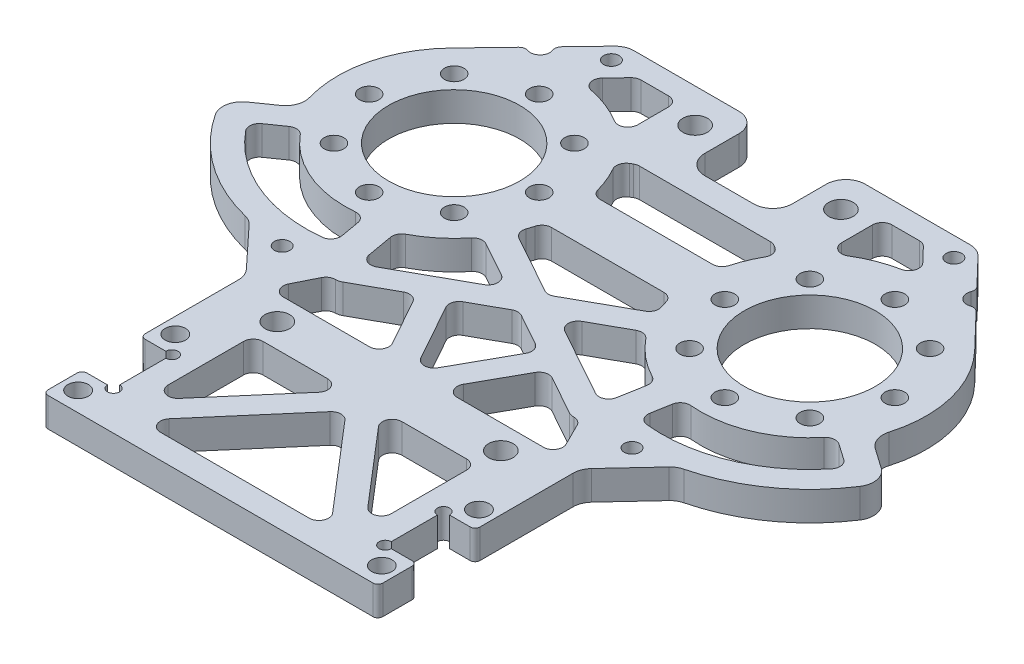
from build123d import *

# Parameters (mm, degrees)
SKETCH1_R              = 13.5
SKETCH1_R_2            = 2.525
SKETCH1_R_3            = 2.01
SKETCH1_R_4            = 2.1
SKETCH1_R_5            = 1.6
BOSS_EXTRUDE1_DEPTH    = 6
CUT_EXTRUDE1_DEPTH     = 111.547291087
R2_CUTOUT_FILLET_R     = 2
R1_PLUG_IN_FILLET_R    = 1
R4_OUTER_EDGE_FILLET_R = 4
F_73_20_MARKING_DEPTH  = 110.7530004


with BuildPart() as part:
    # Sketch1 → Boss-Extrude1 (new body)
    with BuildSketch(Plane(origin=(0, 0, 0), x_dir=(1, 0, 0), z_dir=(0, 1, 0))):
        with BuildLine():
            Line((-36.261062267, 35), (-9, 35))
            Line((-9, 35), (-9, 20))
            Line((-9, 20), (9, 20))
            Line((9, 20), (9, 35))
            Line((9, 35), (36.261062267, 35))
            Line((36.261062267, 35), (53.909452324, 16.624766472))
            ThreePointArc((53.909452324, 16.624766472), (60.203109588, 4.346632924), (58.696156922, -9.368022698))
            Line((58.696156922, -9.368022698), (68.25790113, -16.063228071))
            ThreePointArc((68.25790113, -16.063228071), (58.255238391, -28.130066659), (44.031297301, -34.713481825))
            Line((44.031297301, -34.713481825), (34.45, -45))
            Line((34.45, -45), (34.45, -66.75))
            Line((34.45, -66.75), (29.2, -66.75))
            ThreePointArc((29.2, -66.75), (27.066116524, -65.866116524), (27.95, -68))
            Line((27.95, -68), (27.95, -77.5))
            ThreePointArc((27.95, -77.5), (27.066116524, -79.633883476), (29.2, -78.75))
            Line((29.2, -78.75), (34.45, -78.75))
            Line((34.45, -78.75), (34.45, -86.75))
            Line((34.45, -86.75), (-34.45, -86.75))
            Line((-34.45, -86.75), (-34.45, -78.75))
            Line((-34.45, -78.75), (-29.2, -78.75))
            ThreePointArc((-29.2, -78.75), (-27.066116524, -79.633883476), (-27.95, -77.5))
            Line((-27.95, -77.5), (-27.95, -68))
            ThreePointArc((-27.95, -68), (-27.066116524, -65.866116524), (-29.2, -66.75))
            Line((-29.2, -66.75), (-34.45, -66.75))
            Line((-34.45, -66.75), (-34.45, -45))
            Line((-34.45, -45), (-44.031297301, -34.713481825))
            ThreePointArc((-44.031297301, -34.713481825), (-58.255238391, -28.130066659), (-68.25790113, -16.063228071))
            Line((-68.25790113, -16.063228071), (-58.696156922, -9.368022698))
            ThreePointArc((-58.696156922, -9.368022698), (-60.203109588, 4.346632924), (-53.909452324, 16.624766472))
            Line((-53.909452324, 16.624766472), (-36.261062267, 35))
        make_face()
        with Locations(Location((-36.6, 0, 0), (0, 0, 270))):
            Circle(SKETCH1_R, mode=Mode.SUBTRACT)
        with Locations(Location((-15, 28, 0), (0, 0, 270))):
            Circle(SKETCH1_R_2, mode=Mode.SUBTRACT)
        with Locations(Location((15, 28, 0), (0, 0, 270))):
            Circle(SKETCH1_R_2, mode=Mode.SUBTRACT)
        with Locations(Location((-23, -50, 0), (0, 0, 270))):
            Circle(SKETCH1_R_2, mode=Mode.SUBTRACT)
        with Locations(Location((23, -50, 0), (0, 0, 270))):
            Circle(SKETCH1_R_2, mode=Mode.SUBTRACT)
        with Locations(Location((36.6, 0, 0), (0, 0, 90))):
            Circle(SKETCH1_R, mode=Mode.SUBTRACT)
        with Locations(Location((-36.6, 17.5, 0), (0, 0, 270))):
            Circle(SKETCH1_R_3, mode=Mode.SUBTRACT)
        with Locations(Location((-24.225631329, 12.374368671, 0), (0, 0, 270))):
            Circle(SKETCH1_R_3, mode=Mode.SUBTRACT)
        with Locations(Location((-19.1, 0, 0), (0, 0, 270))):
            Circle(SKETCH1_R_3, mode=Mode.SUBTRACT)
        with Locations(Location((-24.225631329, -12.374368671, 0), (0, 0, 270))):
            Circle(SKETCH1_R_3, mode=Mode.SUBTRACT)
        with Locations(Location((-36.6, -17.5, 0), (0, 0, 270))):
            Circle(SKETCH1_R_3, mode=Mode.SUBTRACT)
        with Locations(Location((-48.974368671, -12.374368671, 0), (0, 0, 270))):
            Circle(SKETCH1_R_3, mode=Mode.SUBTRACT)
        with Locations(Location((-54.1, 0, 0), (0, 0, 270))):
            Circle(SKETCH1_R_3, mode=Mode.SUBTRACT)
        with Locations(Location((-48.974368671, 12.374368671, 0), (0, 0, 270))):
            Circle(SKETCH1_R_3, mode=Mode.SUBTRACT)
        with Locations(Location((48.974368671, 12.374368671, 0), (0, 0, 90))):
            Circle(SKETCH1_R_3, mode=Mode.SUBTRACT)
        with Locations(Location((54.1, 0, 0), (0, 0, 90))):
            Circle(SKETCH1_R_3, mode=Mode.SUBTRACT)
        with Locations(Location((48.974368671, -12.374368671, 0), (0, 0, 90))):
            Circle(SKETCH1_R_3, mode=Mode.SUBTRACT)
        with Locations(Location((36.6, -17.5, 0), (0, 0, 90))):
            Circle(SKETCH1_R_3, mode=Mode.SUBTRACT)
        with Locations(Location((24.225631329, -12.374368671, 0), (0, 0, 90))):
            Circle(SKETCH1_R_3, mode=Mode.SUBTRACT)
        with Locations(Location((19.1, 0, 0), (0, 0, 90))):
            Circle(SKETCH1_R_3, mode=Mode.SUBTRACT)
        with Locations(Location((24.225631329, 12.374368671, 0), (0, 0, 90))):
            Circle(SKETCH1_R_3, mode=Mode.SUBTRACT)
        with Locations(Location((36.6, 17.5, 0), (0, 0, 90))):
            Circle(SKETCH1_R_3, mode=Mode.SUBTRACT)
        with Locations(Location((-31.25, -82.75, 0), (0, 0, 270))):
            Circle(SKETCH1_R_4, mode=Mode.SUBTRACT)
        with Locations(Location((-31.25, -62.75, 0), (0, 0, 270))):
            Circle(SKETCH1_R_4, mode=Mode.SUBTRACT)
        with Locations(Location((31.25, -82.75, 0), (0, 0, 90))):
            Circle(SKETCH1_R_4, mode=Mode.SUBTRACT)
        with Locations(Location((31.25, -62.75, 0), (0, 0, 90))):
            Circle(SKETCH1_R_4, mode=Mode.SUBTRACT)
        with Locations(Location((-35.25, 31, 0), (0, 0, 270))):
            Circle(SKETCH1_R_5, mode=Mode.SUBTRACT)
        with Locations(Location((35.25, 31, 0), (0, 0, 90))):
            Circle(SKETCH1_R_5, mode=Mode.SUBTRACT)
        with Locations(Location((-36, -36, 0), (0, 0, 270))):
            Circle(SKETCH1_R_5, mode=Mode.SUBTRACT)
        with Locations(Location((36, -36, 0), (0, 0, 90))):
            Circle(SKETCH1_R_5, mode=Mode.SUBTRACT)
        with BuildLine():
            Line((-55.030920997, -12.905469818), (-61.584137351, -17.494081309))
            ThreePointArc((-61.584137351, -17.494081309), (-48.271844687, -28.178325742), (-31.303730581, -30.036636467))
            Line((-31.303730581, -30.036636467), (-32.692916002, -22.158174443))
            ThreePointArc((-32.692916002, -22.158174443), (-45.210377228, -20.787289482), (-55.030920997, -12.905469818))
        make_face(mode=Mode.SUBTRACT)
        with BuildLine():
            Line((55.030920997, -12.905469818), (61.584137351, -17.494081309))
            ThreePointArc((61.584137351, -17.494081309), (48.271844687, -28.178325742), (31.303730581, -30.036636467))
            Line((31.303730581, -30.036636467), (32.692916002, -22.158174443))
            ThreePointArc((32.692916002, -22.158174443), (45.210377228, -20.787289482), (55.030920997, -12.905469818))
        make_face(mode=Mode.SUBTRACT)
    extrude(amount=BOSS_EXTRUDE1_DEPTH)

    # Sketch3 → Cut-Extrude1 (cut, through all)
    with BuildSketch(Plane(origin=(0, 6, 0), x_dir=(1, 0, 0), z_dir=(0, 1, 0))):
        with BuildLine():
            Line((-35.748265569, 23.984881664), (-29.490856678, 30.5))
            Line((-29.490856678, 30.5), (-21, 30.5))
            Line((-21, 30.5), (-21, 18.238420984))
            ThreePointArc((-21, 18.238420984), (-27.886771893, 22.362460866), (-35.748265569, 23.984881664))
        make_face()
        with BuildLine():
            ThreePointArc((35.748265569, 23.984881664), (27.886771893, 22.362460866), (21, 18.238420984))
            Line((21, 18.238420984), (21, 30.5))
            Line((21, 30.5), (29.490856678, 30.5))
            Line((29.490856678, 30.5), (35.748265569, 23.984881664))
        make_face()
        with BuildLine():
            Line((-13.126610811, 5), (13.126610811, 5))
            ThreePointArc((13.126610811, 5), (14.513085915, 9.389793725), (16.712198489, 13.434111472))
            Line((16.712198489, 13.434111472), (14, 15))
            Line((14, 15), (-14, 15))
            Line((-14, 15), (-16.712198489, 13.434111472))
            ThreePointArc((-16.712198489, 13.434111472), (-14.513085915, 9.389793725), (-13.126610811, 5))
        make_face()
        with BuildLine():
            Line((13.126610811, -5), (-13.126610811, -5))
            ThreePointArc((-13.126610811, -5), (-13.719828244, -7.245532444), (-14.527321777, -9.423209435))
            ThreePointArc((-14.527321777, -9.423209435), (-14.469211894, -9.452626985), (-14.411888075, -9.483548344))
            Line((-14.411888075, -9.483548344), (0, -17.501639796))
            Line((0, -17.501639796), (14.411888075, -9.483548344))
            ThreePointArc((14.411888075, -9.483548344), (14.469211894, -9.452626985), (14.527321777, -9.423209435))
            ThreePointArc((14.527321777, -9.423209435), (13.719828244, -7.245532444), (13.126610811, -5))
        make_face()
        with BuildLine():
            ThreePointArc((-16.842763472, -13.852855474), (-16.899262321, -13.820451295), (-16.95489785, -13.786586289))
            ThreePointArc((-16.95489785, -13.786586289), (-21.266831345, -18.463313327), (-26.655934481, -21.842975094))
            Line((-26.655934481, -21.842975094), (-24.97170536, -31.394713087))
            Line((-24.97170536, -31.394713087), (-13.806916689, -25.183153842))
            Line((-13.806916689, -25.183153842), (-5.142180472, -20.362505289))
            Line((-5.142180472, -20.362505289), (-16.842763472, -13.852855474))
        make_face()
        with BuildLine():
            ThreePointArc((-23.296885286, -36.184653565), (-24.456132251, -36.499368441), (-25.628351624, -36.237069529))
            Line((-25.628351624, -36.237069529), (-30, -45))
            Line((-30, -45), (-5.642628511, -45))
            Line((-5.642628511, -45), (-13.560695072, -30.767898791))
            Line((-13.560695072, -30.767898791), (-23.296885286, -36.184653565))
        make_face()
        Polygon((9.191387942, -28.337023394), (0, -23.223370782), (-9.191387942, -28.337023394), (0, -44.857819528), align=None)
        with BuildLine():
            ThreePointArc((26.655934481, -21.842975094), (21.266831345, -18.463313327), (16.95489785, -13.786586289))
            ThreePointArc((16.95489785, -13.786586289), (16.899262321, -13.820451295), (16.842763472, -13.852855474))
            Line((16.842763472, -13.852855474), (5.142180472, -20.362505289))
            Line((5.142180472, -20.362505289), (13.806916944, -25.183153984))
            Line((13.806916944, -25.183153984), (24.97170536, -31.394713087))
            Line((24.97170536, -31.394713087), (26.655934481, -21.842975094))
        make_face()
        with BuildLine():
            Line((30, -45), (25.628351624, -36.237069529))
            ThreePointArc((25.628351624, -36.237069529), (24.456132251, -36.499368441), (23.296885286, -36.184653565))
            Line((23.296885286, -36.184653565), (13.560695072, -30.767898791))
            Line((13.560695072, -30.767898791), (5.642628511, -45))
            Line((5.642628511, -45), (30, -45))
        make_face()
        Polygon((-3.29399812, -55), (-22.95, -77.910590426), (-22.95, -55), align=None)
        Polygon((0, -58.839409574), (19.65600188, -81.75), (-19.65600188, -81.75), align=None)
        Polygon((22.95, -55), (3.29399812, -55), (22.95, -77.910590426), align=None)
    extrude(amount=-CUT_EXTRUDE1_DEPTH, mode=Mode.SUBTRACT)

    # R2 cutout fillet
    r2_cutout_fillet_edges = [part.edges().sort_by_distance(p)[0] for p in [
        (-13.126610811, 3, 5),
        (13.126610811, 3, 5),
        (26.655934481, 3, 21.842975094),
        (-26.655934481, 3, 21.842975094),
        (22.95, 3, 55),
        (22.95, 3, 77.910590426),
        (3.29399812, 3, 55),
        (19.65600188, 3, 81.75),
        (-19.65600188, 3, 81.75),
        (0, 3, 58.839409574),
        (-3.29399812, 3, 55),
        (-22.95, 3, 77.910590426),
        (-22.95, 3, 55),
        (-16.712198489, 3, -13.434111472),
        (14, 3, -15),
        (16.712198489, 3, -13.434111472),
        (13.126610811, 3, -5),
        (-13.126610811, 3, -5),
        (-14, 3, -15),
        (21, 3, -30.5),
        (29.490856678, 3, -30.5),
        (35.748265569, 3, -23.984881664),
        (21, 3, -18.238420984),
        (-5.142180472, 3, 20.362505289),
        (-24.97170536, 3, 31.394713087),
        (-16.95489785, 3, 13.786586289),
        (-14.527321777, 3, 9.423209435),
        (14.527321777, 3, 9.423209435),
        (16.95489785, 3, 13.786586289),
        (0, 3, 17.501639796),
        (24.97170536, 3, 31.394713087),
        (5.142180472, 3, 20.362505289),
        (5.642628511, 3, 45),
        (13.560695072, 3, 30.767898791),
        (25.628351624, 3, 36.237069529),
        (30, 3, 45),
        (-13.560695072, 3, 30.767898791),
        (-5.642628511, 3, 45),
        (-30, 3, 45),
        (-25.628351624, 3, 36.237069529),
        (0, 3, 23.223370782),
        (9.191387942, 3, 28.337023394),
        (0, 3, 44.857819528),
        (-9.191387942, 3, 28.337023394),
        (-21, 3, -30.5),
        (-21, 3, -18.238420984),
        (-35.748265569, 3, -23.984881664),
        (61.584137351, 3, 17.494081309),
        (31.303730581, 3, 30.036636467),
        (32.692916002, 3, 22.158174443),
        (55.030920997, 3, 12.905469818),
        (-31.303730581, 3, 30.036636467),
        (-61.584137351, 3, 17.494081309),
        (-55.030920997, 3, 12.905469818),
        (-32.692916002, 3, 22.158174443),
        (-29.490856678, 3, -30.5),
    ]]
    fillet(r2_cutout_fillet_edges, radius=R2_CUTOUT_FILLET_R)

    # R1 plug-in fillet
    r1_plug_in_fillet_edges = [part.edges().sort_by_distance(p)[0] for p in [
        (34.45, 3, 86.75),
        (-34.45, 3, 86.75),
        (-34.45, 3, 78.75),
        (-34.45, 3, 66.75),
        (34.45, 3, 66.75),
        (34.45, 3, 78.75),
    ]]
    fillet(r1_plug_in_fillet_edges, radius=R1_PLUG_IN_FILLET_R)

    # R4 outer edge fillet
    r4_outer_edge_fillet_edges = [part.edges().sort_by_distance(p)[0] for p in [
        (-34.45, 3, 45),
        (-44.031297301, 3, 34.713481825),
        (-68.25790113, 3, 16.063228071),
        (-58.696156922, 3, 9.368022698),
        (-36.261062267, 3, -35),
        (-9, 3, -35),
        (-9, 3, -20),
        (9, 3, -20),
        (9, 3, -35),
        (36.261062267, 3, -35),
        (58.696156922, 3, 9.368022698),
        (68.25790113, 3, 16.063228071),
        (44.031297301, 3, 34.713481825),
        (34.45, 3, 45),
    ]]
    fillet(r4_outer_edge_fillet_edges, radius=R4_OUTER_EDGE_FILLET_R)

    # Sketch4 → 73.20 marking (cut, through all)
    with BuildSketch(Plane(origin=(0, 6, 0), x_dir=(1, 0, 0), z_dir=(0, 1, 0))):
        with BuildLine():
            Line((-42.714556509, 28.2807206), (-47.095567144, 23.7192794))
            ThreePointArc((-47.095567144, 23.7192794), (-46.372654237, 24.136655469), (-45.538584425, 24.102989426))
            ThreePointArc((-45.538584425, 24.102989426), (-43.462607466, 24.614602794), (-43.035149776, 26.709527254))
            ThreePointArc((-43.035149776, 26.709527254), (-43.102432535, 27.541560237), (-42.714556509, 28.2807206))
        make_face()
        with BuildLine():
            Line((42.714556509, 28.2807206), (47.095567144, 23.7192794))
            ThreePointArc((47.095567144, 23.7192794), (46.372654237, 24.136655469), (45.538584425, 24.102989426))
            ThreePointArc((45.538584425, 24.102989426), (43.462607466, 24.614602794), (43.035149776, 26.709527254))
            ThreePointArc((43.035149776, 26.709527254), (43.102432535, 27.541560237), (42.714556509, 28.2807206))
        make_face()
    extrude(amount=-F_73_20_MARKING_DEPTH, mode=Mode.SUBTRACT)


solid = part.part
